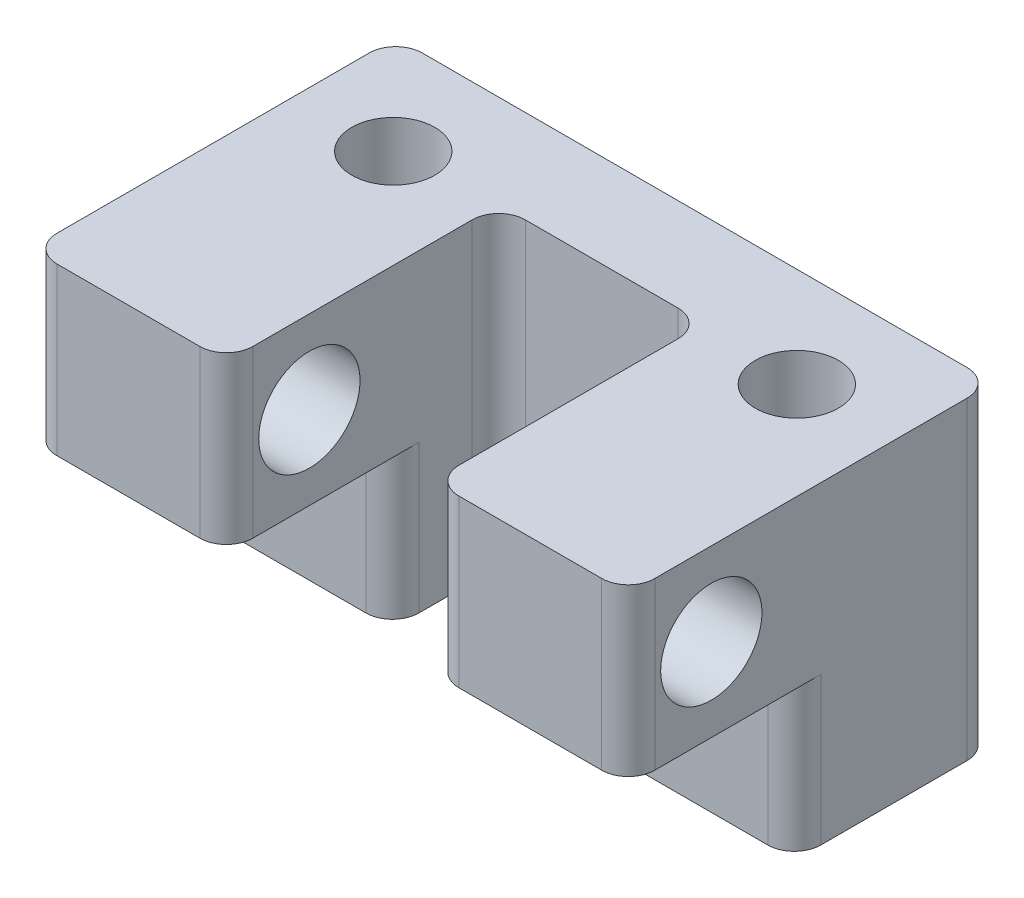
from build123d import *

# Parameters (mm, degrees)
EXTRUDE_1_DEPTH     = 4.45
EXTRUDE_2_DEPTH     = 5
HOLE_WIZARD_M3_1_D  = 2.5
SKETCH_5_R          = 1.525
CUT_EXTRUDE_1_DEPTH = 22.921279616
FILLET_R0_8_1_R     = 0.8


with BuildPart() as part:
    # 草图1 → 凸台-拉伸1 (new body)
    with BuildSketch(Plane(origin=(0, 0, 0), x_dir=(1, 0, 0), z_dir=(0, 1, 0))):
        Polygon((-9, 2.8), (9, 2.8), (9, -3.2), (3.1, -3.2), (3.1, 0), (-3.1, 0), (-3.1, -3.2), (-9, -3.2), align=None)
    extrude(amount=EXTRUDE_1_DEPTH)

    # 草图2 → 凸台-拉伸2 (add)
    with BuildSketch(Plane(origin=(0, 4.45, 0), x_dir=(1, 0, 0), z_dir=(0, 1, 0))):
        Polygon((-3.1, -8.2), (-3.1, 0), (3.1, 0), (3.1, -8.2), (9, -8.2), (9, 2.8), (-9, 2.8), (-9, -8.2), align=None)
    extrude(amount=EXTRUDE_2_DEPTH)

    # M3 螺纹孔1 (through all)
    with Locations(Plane.XZ):
        with Locations((-6.075, 0.2), (6.075, 0.2)):
            Hole(HOLE_WIZARD_M3_1_D / 2)

    # 草图5 → 切除-拉伸1 (cut, through all)
    with BuildSketch(Plane.ZY.offset(9)):
        with Locations((5.7, 6.95)):
            Circle(SKETCH_5_R)
    extrude(amount=-CUT_EXTRUDE_1_DEPTH, mode=Mode.SUBTRACT)

    # R0.8 圆角1
    fillet_r0_8_1_edges = [part.edges().sort_by_distance(p)[0] for p in [
        (-9, 4.725, -2.8),
        (9, 4.725, -2.8),
        (9, 2.225, 3.2),
        (3.1, 2.225, 3.2),
        (3.1, 4.725, 0),
        (-3.1, 4.725, 0),
        (-3.1, 2.225, 3.2),
        (-9, 2.225, 3.2),
        (-9, 6.95, 8.2),
        (-3.1, 6.95, 8.2),
        (3.1, 6.95, 8.2),
        (9, 6.95, 8.2),
    ]]
    fillet(fillet_r0_8_1_edges, radius=FILLET_R0_8_1_R)


solid = part.part
